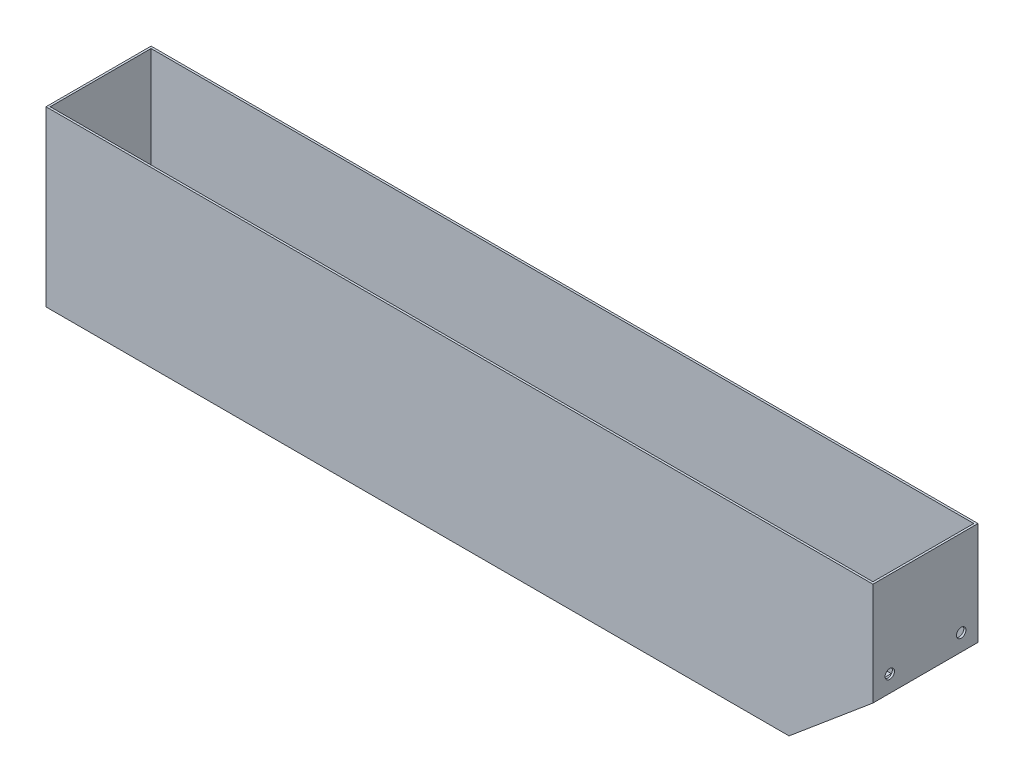
SolidWorks part; units mm, degrees
ref_plane "前视基准面" through (0, 0, 0) normal (0, 0, 1) x (1, 0, 0)
ref_plane "上视基准面" through (0, 0, 0) normal (0, 1, 0) x (1, 0, 0)
ref_plane "右视基准面" through (0, 0, 0) normal (1, 0, 0) x (0, 0, -1)
sketch "草图1" plane through (0, 0, 0) normal (0, 0, 1) x (1, 0, 0)
  line L0 (0, 0) -> (707.1525, 0)
  line L1 (707.1525, 0) -> (787, 67)
  line L2 (787, 67) -> (787, 165)
  line L3 (787, 165) -> (0, 165)
  line L4 (0, 165) -> (0, 0)
  dimension "D1" = 787
  dimension "D2" = 140
  dimension "D3" = 165
  dimension "D4" = 67
extrude "凸台-拉伸1" add sketch "草图1" along normal blind 100
shell "抽壳1" thickness 2
sketch "草图2" plane through (0, 0, 0) normal (-1, 0, 0) x (0, 0, 1)
  line L1 (0, 165) -> (0, 0) construction
  line L2 (100, 16) -> (0, 16)
  line L3 (100, 16) -> (0, 16) construction
  line L4 (100, 165) -> (100, 0) construction
  circle A0 centre (16, 16) radius 4.5
  circle A1 centre (84, 16) radius 4.5
  dimension "D2" = 9
  dimension "D3" = 9
  dimension "D4" = 16
  dimension "D5" = 16
  dimension "D1" = 16
extrude "切除-拉伸1" cut sketch "草图2" against normal blind 10
sketch "草图3" plane through (787, 0, 0) normal (1, 0, 0) x (0, 0, -1)
  line L0 (-84, 83) -> (-16, 83) construction
  line L1 (-100, 67) -> (0, 67) construction
  line L2 (-100, 67) -> (-100, 165) construction
  line L3 (0, 67) -> (0, 165) construction
  circle A0 centre (-84, 83) radius 4.5
  circle A1 centre (-16, 83) radius 4.5
  dimension "D2" = 9
  dimension "D3" = 9
  dimension "D4" = 16
  dimension "D5" = 16
  dimension "D1" = 16
extrude "切除-拉伸2" cut sketch "草图3" against normal blind 10
